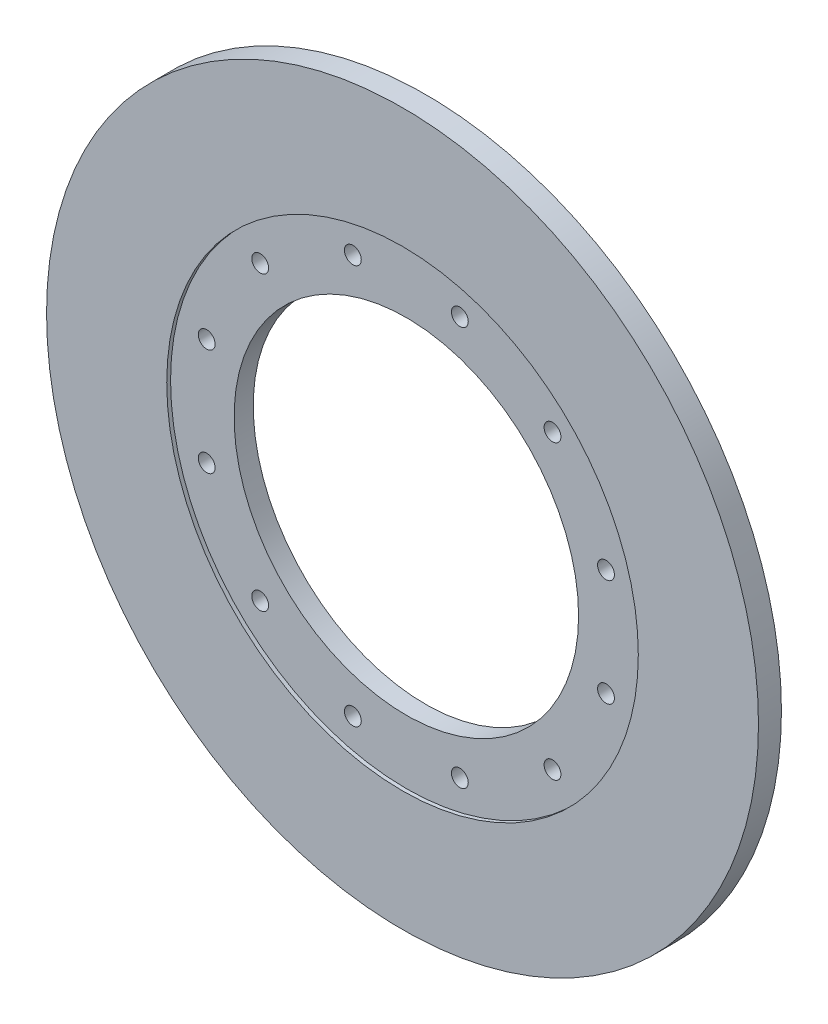
SolidWorks part; units mm, degrees
material "Q235"
ref_plane "Front Plane" through (0, 0, 0) normal (0, 0, 1) x (1, 0, 0)
ref_plane "Top Plane" through (0, 0, 0) normal (0, 1, 0) x (1, 0, 0)
ref_plane "Right Plane" through (0, 0, 0) normal (1, 0, 0) x (0, 0, -1)
sketch "Sketch1" plane through (0, 0, 0) normal (0, 0, 1) x (1, 0, 0)
  circle A0 centre (0, 0) radius 465
  circle A1 centre (0, 0) radius 225
  dimension "D1" = 930
  dimension "D2" = 450
extrude "Boss-Extrude1" add sketch "Sketch1" along normal blind 30
sketch "Sketch2" plane through (0, 0, 30) normal (0, 0, 1) x (1, 0, 0)
  circle A0 centre (0, 0) radius 308
  dimension "D1" = 616
extrude "Cut-Extrude1" cut sketch "Sketch2" against normal blind 5
sketch "Sketch4" plane through (0, 0, 0) normal (0, 0, -1) x (-1, 0, 0)
  line L0 (-465, 0) -> (465, 0) construction
  line L1 (0, 0) -> (-449.1555, 120.3509) construction
  circle A0 centre (0, 0) radius 465 construction
  circle A1 centre (0, 0) radius 270 construction
  circle A2 centre (-260.8, 69.8811) radius 11
  circle A3 centre (-190.9188, 190.9188) radius 11
  circle A4 centre (-69.8811, 260.8) radius 11
  circle A5 centre (69.8811, 260.8) radius 11
  circle A6 centre (190.9188, 190.9188) radius 11
  circle A7 centre (260.8, 69.8811) radius 11
  circle A8 centre (260.8, -69.8811) radius 11
  circle A9 centre (190.9188, -190.9188) radius 11
  circle A10 centre (69.8811, -260.8) radius 11
  circle A11 centre (-69.8811, -260.8) radius 11
  circle A12 centre (-190.9188, -190.9188) radius 11
  circle A13 centre (-260.8, -69.8811) radius 11
  point P35 (0, 0)
  dimension "D1" = 540
  dimension "D3" = 22
  dimension "D2" = 15
  dimension "D4" = 12
extrude "Cut-Extrude7" cut sketch "Sketch4" against normal through all both and the other way through all
sketch "Sketch5" plane through (0, 0, 0) normal (0, 0, -1) x (-1, 0, 0)
  line L0 (0, 465) -> (0, 0) construction
  circle A0 centre (0, 0) radius 465 construction
sketch "Sketch6" plane through (0, 0, 30) normal (0, 0, 1) x (1, 0, 0)
  line L1 (0, 0) -> (188.9851, 327.3317) construction
  line L2 (0, 465) -> (0, 0) construction
  dimension "D1" = 30
